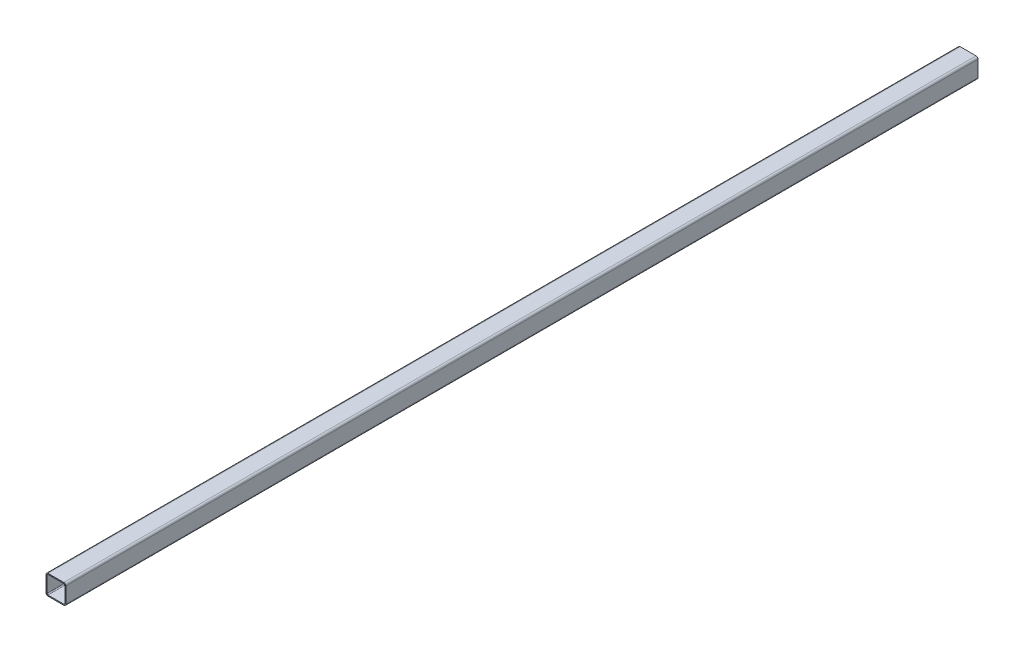
SolidWorks part; units mm, degrees
material "普通碳钢"
ref_plane "Front Plane" through (0, 0, 0) normal (0, 0, 1) x (1, 0, 0)
ref_plane "Top Plane" through (0, 0, 0) normal (0, 1, 0) x (1, 0, 0)
ref_plane "Right Plane" through (0, 0, 0) normal (1, 0, 0) x (0, 0, -1)
sketch "Sketch1" plane through (0, 0, 0) normal (0, 0, 1) x (1, 0, 0)
  line L0 (10, 95) -> (90, 95)
  line L1 (10, 0) -> (90, 0)
  line L2 (0, 10) -> (0, 90)
  line L3 (10, 100) -> (90, 100)
  line L4 (100, 10) -> (100, 90)
  line L5 (95, 10) -> (95, 90)
  line L6 (10, 5) -> (90, 5)
  line L7 (5, 10) -> (5, 90)
  arc A0 (100, 10) -> (90, 0) centre (90, 10) cw
  arc A1 (0, 90) -> (10, 100) centre (10, 90) cw
  arc A2 (100, 90) -> (90, 100) centre (90, 90) ccw
  arc A3 (10, 0) -> (0, 10) centre (10, 10) cw
  arc A4 (95, 90) -> (90, 95) centre (90, 90) ccw
  arc A5 (95, 10) -> (90, 5) centre (90, 10) cw
  arc A6 (10, 5) -> (5, 10) centre (10, 10) cw
  arc A7 (5, 90) -> (10, 95) centre (10, 90) cw
  point P7 (100, 0)
  point P10 (0, 100)
  point P13 (100, 100)
  point P16 (0, 0)
  dimension "D3" = 10
  dimension "D4" = 10
  dimension "D5" = 10
  dimension "D6" = 10
  dimension "D1" = 100
  dimension "D2" = 100
  dimension "D7" = 5
extrude "Boss-Extrude1" add sketch "Sketch1" along normal blind 4600
